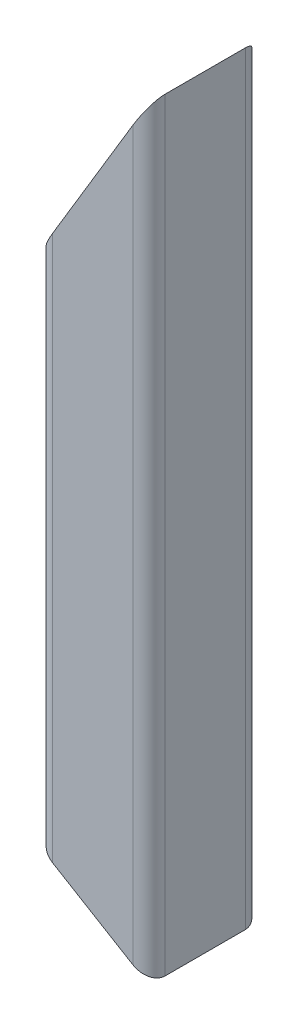
from build123d import *

# Parameters (mm, degrees)
GB_T6728_2002_70_70_5_1_DEPTH = 476
CUT_EXTRUDE_1_DEPTH           = 483.390920313
CUT_EXTRUDE_1_DEPTH_BACK      = 483.390920313


with BuildPart() as part:
    # Sketch1 → 结构用冷弯空心方钢(gb t6728-2002) 70×70×5(1) (new body)
    with BuildSketch(Plane(origin=(0, 0, 0), x_dir=(-1, 0, 0), z_dir=(0, 1, 0))):
        with BuildLine():
            Line((-25, -35), (25, -35))
            ThreePointArc((25, -35), (32.071067812, -32.071067812), (35, -25))
            Line((35, -25), (35, 25))
            ThreePointArc((35, 25), (32.071067812, 32.071067812), (25, 35))
            Line((25, 35), (-25, 35))
            ThreePointArc((-25, 35), (-32.071067812, 32.071067812), (-35, 25))
            Line((-35, 25), (-35, -25))
            ThreePointArc((-35, -25), (-32.071067812, -32.071067812), (-25, -35))
        make_face()
        with BuildLine():
            Line((-25, -30), (25, -30))
            ThreePointArc((25, -30), (28.535533906, -28.535533906), (30, -25))
            Line((30, -25), (30, 25))
            ThreePointArc((30, 25), (28.535533906, 28.535533906), (25, 30))
            Line((25, 30), (-25, 30))
            ThreePointArc((-25, 30), (-28.535533906, 28.535533906), (-30, 25))
            Line((-30, 25), (-30, -25))
            ThreePointArc((-30, -25), (-28.535533906, -28.535533906), (-25, -30))
        make_face(mode=Mode.SUBTRACT)
    extrude(amount=GB_T6728_2002_70_70_5_1_DEPTH)

    # 草图2 → 切除-拉伸1 (cut, two sides: drawn at the far end of the back side and taken through both)
    with BuildSketch(Plane.XY.offset(35).offset(-CUT_EXTRUDE_1_DEPTH_BACK)):
        Polygon((35, 476), (-35, 359.333333333), (-35, 476), align=None)
        Polygon((-35, 42), (35, 0), (-35, 0), align=None)
    extrude(amount=CUT_EXTRUDE_1_DEPTH + CUT_EXTRUDE_1_DEPTH_BACK, mode=Mode.SUBTRACT)


solid = part.part
